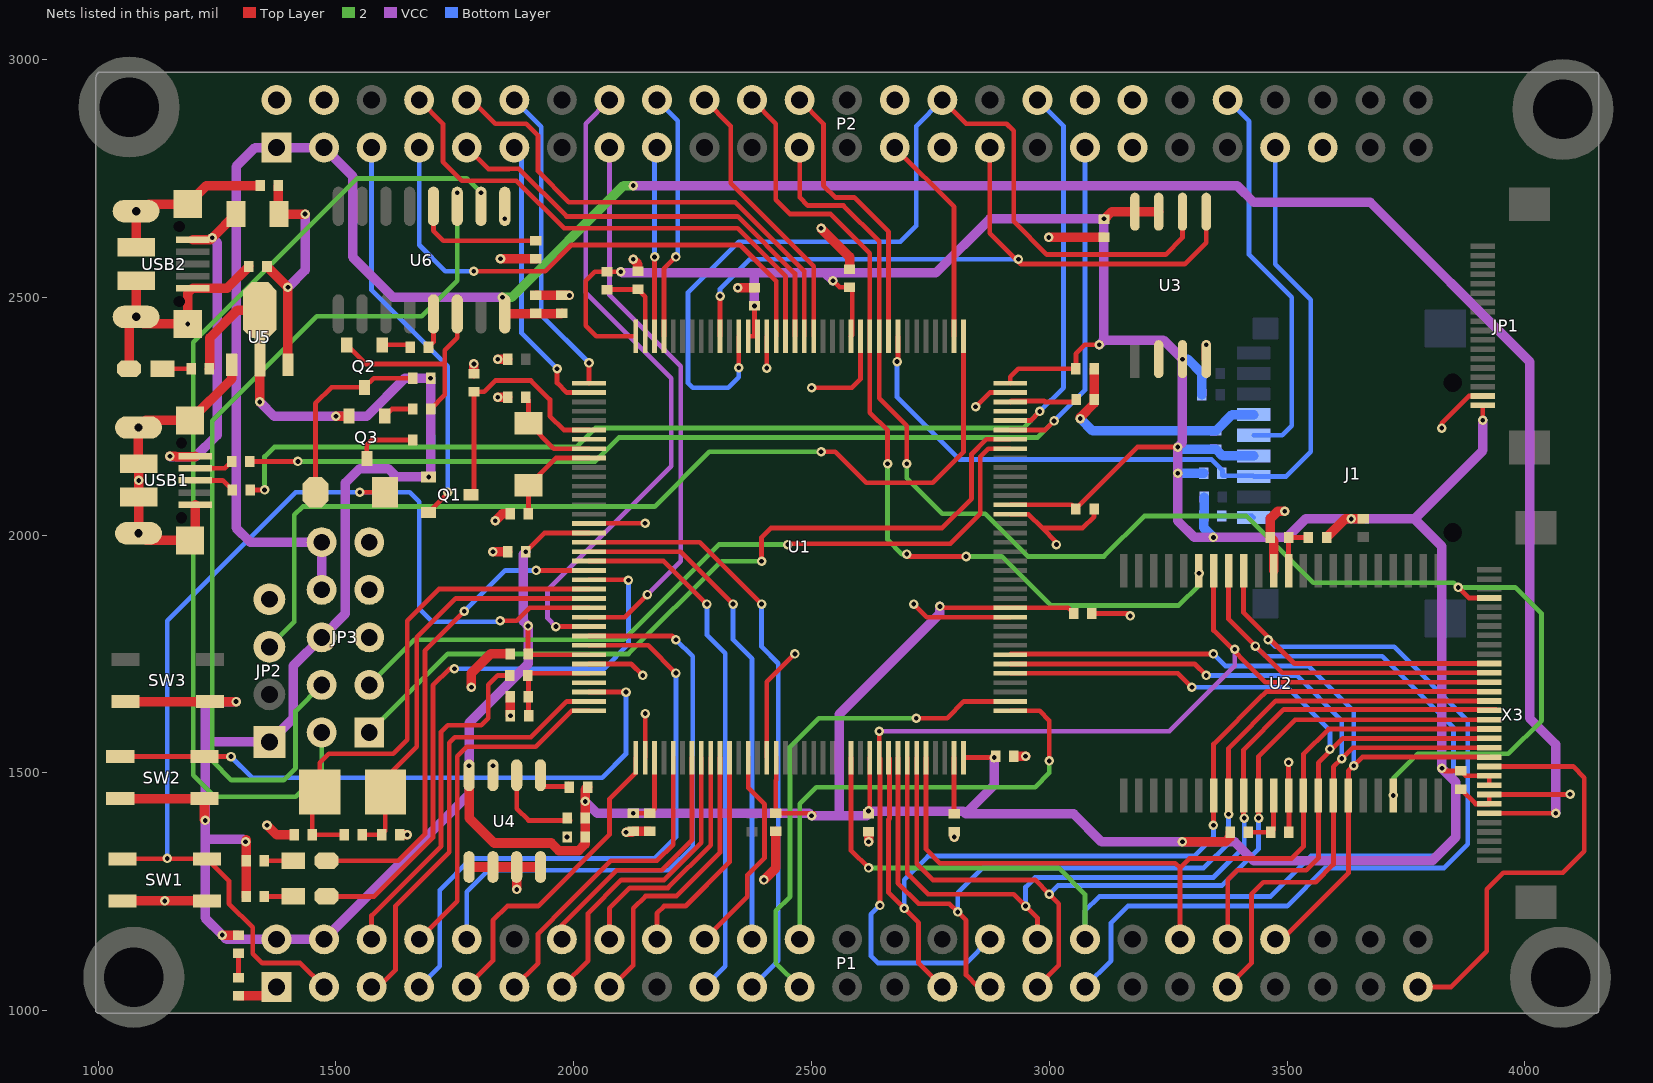
[diagram p0: the nets of this part, all layers, seen from the top]
# Altium PCB MISC105440.PcbDoc (part 2 of 2)
Units mil, origin at the board's own origin, x right, y up, seen from the top; angles counter-clockwise.
Board outline 3160.03 x 1978.53 mil, 4 copper layers (Top Layer, 2, VCC, Bottom Layer), stack 30.634 mil thick; 91 components, 148 nets, 590 pads, 216 vias.

## Via types
v1: diameter 20, hole 10, Top Layer to Bottom Layer, 216 vias

## Nets (pads, with @x,y where several pads share a name; then routed paths per layer and width w, separated by ;. In a path a pad name is that pad's centre, name@x,y a point inside that pad or via, vN(x,y) a via of type N, cw(c..) or ccw(c..) an arc to the next point about the centre after c; other vN are vias at no path point) (continued)
FSMC_D5: P1.35 U2.14 X3.22 | length 2375.7
  Top Layer w10: U2.14@3408.5,1925 3408.5,1836.5 3515,1730 X3.22@3925,1730
  Bottom Layer w10: P1.35@3075,1050 3130,1105 3130,1185 3165,1220 3500,1220 3580,1300 3830,1300 3880,1350 3880,1610 3725,1765 3475,1765 v1(3460,1780)
FSMC_D6: P1.36 U1.60 U2.15 X3.21 | length 3139.6
  Top Layer w10: U1.60@2583.27,1532.09 2583.27,1336.73 v1(2620,1300) ; U2.15@3377.01,1925 3377.01,1822.99 3489.69,1710.31 X3.21@3925,1710.31
  2 w10: v1(2620,1300) 3020,1300 3075,1245 P1.36@3075,1150
  Bottom Layer w10: P1.36@3075,1150 3075,1210 3105,1240 3465,1240 3550,1325 3820,1325 3850,1355 3850,1595 3700,1745 3455,1745 v1(3433.35,1766.65)
FSMC_D7: P1.32 U1.63 U2.16 X3.20 | length 2349.3
  Top Layer w10: v1(2642.32,1587.68) U1.63@2642.32,1532.09 2643.81,1530.6 v1(2643.81,1221.19) v1@2645,1220 ; U2.16@3345.51,1925 3345.51,1799.49 3454.37,1690.63 X3.20@3925,1690.63
  VCC w10: v1(2642.32,1587.68) 3252.68,1587.68 3390,1725 v1(3390,1760)
  Bottom Layer w10: v1(2643.81,1221.19) 2625,1202.38 2625,1115 2640,1100 2825,1100 P1.32@2875,1150
FSMC_D8: P1.29 U1.64 U2.29 X3.19 | length 2098.8
  Top Layer w10: U1.64@2662.01,1532.09 2664,1530.09 2664,1403.85 2662.01,1401.85 2662.01,1247.99 v1(2695,1215) 2725,1185 2725,1100 P1.29@2775,1050 ; v1(3345,1390) 3345.51,1390.51 U2.29@3345.51,1452.56 3345.51,1560.51 3448,1663 3448.54,1663 3456.48,1670.94 X3.19@3925,1670.94
  Bottom Layer w10: v1(2695,1215) 2695,1275 2745,1325 3305,1325 3345,1365 v1(3345,1390)
FSMC_D9: P1.31 U1.65 U2.30 X3.18 | length 2059.3
  Top Layer w10: U1.65@2681.69,1532.09 2681.69,1268.31 2725,1225 2790,1225 v1(2807.5,1207.5) 2825,1190 2825,1075 2850,1050 P1.31@2875,1050 ; v1(3377.01,1412.99) U2.30@3377.01,1452.56 3377.01,1552.01 3476.26,1651.26 X3.18@3925,1651.26
  Bottom Layer w10: v1(2807.5,1207.5) 2807.5,1247.5 2860,1300 3325,1300 3380,1355 3377.01,1357.99 v1(3377.01,1412.99)
FSMC_D10: P1.34 U1.66 U2.31 X3.17 | length 1906.8
  Top Layer w10: U1.66@2701.38,1532.09 2701.38,1288.62 2745,1245 2925,1245 v1(2950,1220) 2975,1195 P1.34@2975,1150 ; v1(3410,1405) 3408.5,1406.5 U2.31@3408.5,1452.56 3408.5,1548.5 3493.35,1633.35 X3.17@3940,1633.35
  Bottom Layer w10: v1(2950,1220) 2950,1260 2970,1280 3345,1280 3410,1345 v1(3410,1405)
FSMC_D11: P1.33 U1.67 U2.32 X3.16 | length 1941.7
  Top Layer w10: U1.67@2721.06,1532.09 2721.06,1308.94 2755,1275 2970,1275 v1(3000,1245) 3020,1225 3020,1095 P1.33@2975,1050 ; v1(3440,1405) U2.32@3440,1452.56 3440,1535 3516.89,1611.89 X3.16@3925,1611.89
  Bottom Layer w10: v1(3000,1245) 3018,1263 3363,1263 3440,1340 v1(3440,1405)
FSMC_D12: P1.40 U1.68 U2.35 X3.15 | length 1778.6
  Top Layer w10: U1.68@2740.75,1532.09 2740.75,1339.25 2770,1310 3265,1310 3275,1300 ; P1.40@3275,1150 3275,1300 ; X3.15@3925,1592.2 3587.2,1592.2 3534.49,1539.49 U2.35@3534.49,1452.56 3534.49,1344.49 3510,1320 3295,1320 3275,1300
FSMC_D13: P1.42 U1.77 U2.36 X3.14 | length 1677.2
  Top Layer w10: U1.77@2917.91,1709.25 2918.28,1709.62 3270.38,1709.62 v1(3300,1680) ; P1.42@3375,1150 3375,1275 3395,1295 3540,1295 3565.98,1320.98 U2.36@3565.98,1452.56 3565.98,1520.98 3617.52,1572.52 X3.14@3925,1572.52
  Bottom Layer w10: v1(3300,1680) 3500,1680 3590,1590 v1(3590,1550)
FSMC_D14: P1.41 U1.78 U2.37 X3.13 | length 1789.7
  Top Layer w10: U1.78@2917.91,1728.94 3306.06,1728.94 v1(3330,1705) ; P1.41@3375,1050 3425,1100 3425,1245 3450,1270 3560,1270 3597.48,1307.48 U2.37@3597.48,1452.56 3597.48,1512.48 v1(3615,1530) 3637.83,1552.83 X3.13@3925,1552.83
  Bottom Layer w10: v1(3330,1705) 3520,1705 3615,1610 v1(3615,1530)
FSMC_D15: P1.44 U1.79 U2.38 X3.12 | length 1622
  Top Layer w10: U1.79@2917.91,1748.62 2919.29,1750 v1(3345,1750) ; P1.44@3475,1150 3490,1150 3628.98,1288.98 U2.38@3628.98,1452.56 3628.98,1503.98 v1(3640,1515) 3658.15,1533.15 X3.12@3925,1533.15
  Bottom Layer w10: v1(3345,1750) 3370,1725 3545,1725 3640,1630 v1(3640,1515)
FSMC_NBL0: P2.18 U1.141 | length 527.1
  Top Layer w10: U1.141@2189.57,2417.91 2189.57,2559.57 v1(2215,2585)
  Bottom Layer w10: P2.18@2175,2915 2218.5,2871.5 2218.5,2588.5 v1(2215,2585)
FSMC_NBL1: P2.17 U1.142 | length 399.2
  Top Layer w10: U1.142@2169.88,2417.91 v1(2169.88,2584.88)
  Bottom Layer w10: v1(2169.88,2584.88) 2169.88,2809.88 P2.17@2175,2815
FSMC_NE3: P2.20 U1.125 | length 592.2
  Top Layer w10: P2.20@2275,2915 2330,2860 2330,2740 2504.53,2565.47 U1.125@2504.53,2417.91
FSMC_NE4: P2.9 U1.127 | length 932.1
  Top Layer w10: P2.9@1775,2815 1820,2770 1864.14,2770 1864.34,2770.2 1884.8,2770.2 1985,2670 2345,2670 2465.16,2549.84 U1.127@2465.16,2417.91
FSMC_NOE: P2.23 U1.118 U2.41 X3.29 | length 3052.6
  Top Layer w10: P2.23@2475,2815 2475,2710 2492,2693 2567,2693 2642.32,2617.68 U1.118@2642.32,2417.91 2642.32,2287.68 2700,2230 v1(2700,2150) ; v1(3860,1890) 3882.2,1867.8 X3.29@3925,1867.8
  2 w10: v1(2700,2150) 2700,2120 2775,2045 2865,2045 2955,1955 3115,1955 3200,2040 3415,2040 3555,1900 3850,1900 v1(3860,1890) 3980,1890 4035,1835 4035,1610 3965,1540 3775,1540 3723.47,1488.47 v1(3723.47,1452.56)
FSMC_NWE: P2.22 U1.119 U2.17 | length 1847.8
  Top Layer w10: P2.22@2375,2915 2425,2865 2425,2705 2455,2675 2540,2675 2622.64,2592.36 U1.119@2622.64,2417.91 2622.64,2257.36 2660,2220 v1(2660,2150) ; v1(2700,1960) 2705,1955 v1(2825,1955)
  2 w10: v1(2660,2150) 2660,1990 2690,1960 v1(2700,1960) ; v1(2825,1955) 2900,1955 3003,1852 3272,1852 3315,1895 v1(3315,1920)
GND: C1.1 C2.1 C3.1 C4.1 C5.2 C6.2 C9.1 C10.1 C11.1 C12.1 C13.1 C14.1 C15.1 C16.1 C17.1 C18.1 C19.1 C20.1 C21.2 C22.2 C23.2 C24.1 C25.2 C26.2 C27.2 C28.1 C29.1 C30.1 C31.1 C34.2 C35.2 C37.1 C38.1 J1.6 JP1.2 JP2.4 JP3.5 JP3.7 JP3.9 LED3.2 P1.1 P2.2 P2.4 R3.2 R7.1 SW1.2 U1.16 U1.31 U1.38 U1.51 U1.83 U1.94 U1.107 U1.120 U1.130 U2.12 U2.34 U3.4 U4.1 U4.2 U4.3 U4.4 U4.7 U5.1 U6.1 USB1.5 USB2.5 X3.7 X3.8 | length 5765.5
  Top Layer w10: U1.31@2032.09,1728.94 2121.06,1728.94 v1(2145,1705) ; U1.16@2032.09,2024.21 2032.87,2025 v1(2150,2025) ; U1.38@2150.2,1532.09 v1(2150.2,1624.8) ; U1.51@2406.1,1532.09 2406.1,1691.1 v1(2465,1750) ; v1(2406.1,2351.1) U1.130@2406.1,2417.91 ; v1(2500,2310) 2585,2310 2602.95,2327.95 U1.120@2602.95,2417.91 ; v1(2715,1855) 2742.64,1827.36 U1.83@2917.91,1827.36 ; v1(2845,2270) 2874.8,2299.8 U1.107@2917.91,2299.8 ; U1.94@2917.91,2043.9 2956.1,2043.9 2985,2015 ; v1(3015,1980) 3015,1985 2985,2015 ; C14.1@3089.59,1835 3165,1835 v1(3170,1830) ; C18.1@3094,2055 3094,2039 3070,2015 2985,2015 ; v1@3500,1525 v1(3502.99,1522.01) U2.34@3502.99,1452.56 3504,1451.55 C25.2@3504,1375 ; v1(3825,2225) 3825,2235 3882.36,2292.36 JP1.2@3911.69,2292.36 ; C37.1@3865,1466 3896.28,1434.72 X3.7@3925,1434.72 X3.8@3925,1454.41 4094.41,1454.41 v1(4095,1455)
  Top Layer w20: SW1.2@1051.42,1230.71 SW1.2@1228.58,1230.71 ; LED3.2@1065,2350 1065,2444 USB2.5@1079.78,2458.78 ; USB2.5@1080.4,2535 1079.78,2534.38 USB2.5@1079.78,2458.78 ; USB2.5@1080.4,2605 1080.4,2670 1106.39,2695.98 USB2.5@1188.43,2695.98 1227.44,2735 C31.1@1341,2735 ; USB1.5@1203.94,2064 1203.94,1999.53 USB1.5@1193.43,1989.02 1100.79,1989.02 1085.4,2004.4 USB1.5@1085.4,2080 USB1.5@1085.4,2150 1084.78,2150.62 USB1.5@1084.78,2226.22 1099.54,2240.98 USB1.5@1193.43,2240.98 1280.94,2328.5 U5.1@1280.94,2358.07 ; C23.2@1295,1031.59 1356.59,1031.59 P1.1@1375,1050 ; C30.1@1317,2565 1271,2519 USB2.5@1198.94,2519 1188.43,2508.49 v1(1188.43,2444.02) 1094.54,2444.02 USB2.5@1079.78,2458.78 ; v1(1355,1390) 1375,1370 C4.1@1412,1370 ; C3.1@1634,1370 v1(1650,1370) ; U4.1@1780,1302.09 U4.2@1830,1302.09 U4.3@1880,1302.09 ; v1(1785,1680) 1785,1710 1825,1750 C11.1@1866,1750 ; C24.1@1790,2339.59 v1(1790,2360) ; v1(1830,1965) C15.1@1861,1965 ; v1(1835,2030) 1850,2045 C1.1@1866,2045 ; v1(1840,2290) C2.1@1861,2290 ; v1(1840,2370) R7.1@1861,2370 ; v1(1846,2581) C38.1@1920,2581 ; C21.2@1866,1660 1867,1659 v1(1867,1620) ; v1(1880,1255) U4.3@1880,1302.09 ; C35.2@1920,2504 C34.2@1975,2504 v1(1991,2504) ; U4.4@1930,1302.09 U4.3@1880,1302.09 ; v1(2110,1375) 2123,1375 C20.1@2125,1377 C9.1@2160,1377 ; v1(2125,2580) 2135,2570 R3.2@2135,2554.59 ; v1(2345,2520) C13.1@2380,2520 ; v1(2400,1275) 2425,1300 C19.1@2425,1377 ; v1(2520,2645) 2580,2585 C10.1@2580,2559 ; v1(2620,1355) C17.1@2620,1376 ; v1(2800,1365) C5.2@2800,1376 ; C16.1@2925,1535 v1(2950,1535) ; v1(2999,2626) C27.2@3115,2626 ; v1(3065,2245) 3065,2247.56 3094.59,2277.15 C6.2@3094.59,2285 3094,2285.6 C12.1@3094,2350 ; U3.4@3330,2370 v1(3330,2400) ; U2.12@3471.5,1925 3471.5,1988.5 C26.2@3465,1995 3465,2035 3480,2050 v1(3495,2050)
  Bottom Layer w20: v1(3065,2245) 3091,2219 C28.1@3350,2219 3384.31,2253.31 J1.6@3430,2253.31
  other v1: 1140,1230.71 1986,1365 1830,1515 1085.4,2115 1855,2665
IIC_SCL: R15.1 U4.6 | length 173.8
  Top Layer w10: U4.6@1880,1476.46 1880,1425 1905,1400 R15.1@1992,1400
IIC_SDA: R16.1 U4.5 | length 61.6
  Top Layer w10: U4.5@1935,1471.46 R16.1@1989.54,1471.46 ; R16.1@1989.54,1476.46 R16.1@1989.54,1471.46 ; R16.1@1991,1470 R16.1@1989.54,1471.46
LCD_BL: P1.49 X3.11 | length 908.9
  Top Layer w10: P1.49@3775,1050 3845,1050 3920,1125 3920,1255 3955,1290 4080,1290 4125,1335 4125,1490 4101.54,1513.46 X3.11@3925,1513.46
LED0: LED1.2 U1.21 | length 1032.3
  Top Layer w10: LED1.2@1480,1315 1630.96,1315 1687,1371.04 1687,1757 v1(1770,1840) ; v1@1920,1925 v1(1920.79,1925.79) U1.21@2032.09,1925.79
  Bottom Layer w10: v1(1770,1840) 1855.79,1925.79 v1(1920.79,1925.79)
LED1: LED2.2 U1.22 | length 1260.2
  Top Layer w10: LED2.2@1480,1240.26 1580.26,1240.26 1704,1364 1704,1684 1739,1719 v1(1749,1719) ; U1.22@2032.09,1906.1 2113.9,1906.1 v1(2115,1905)
  Bottom Layer w10: v1(1749,1719) 2064,1719 2115,1770 v1(2115,1905)
NetC1_2: C1.2 U1.9 X2.2 | length 211.1
  Top Layer w10: C1.2@1904,2045 1905,2046 X2.2@1905,2105.04 1961.97,2162.01 U1.9@2032.09,2162.01
NetC2_2: C2.2 U1.8 X2.1 | length 206.7
  Top Layer w10: C2.2@1899,2290 1905,2284 X2.1@1905,2234.96 1958.27,2181.69 U1.8@2032.09,2181.69
NetC3_2: C3.2 R1.1 U1.24 X1.1 | length 882.6
  Top Layer w10: R1.1@1555,1370 C3.2@1596,1370 1603.9,1377.9 X1.1@1603.9,1460 1603.9,1488.9 1670,1555 1670,1785 1751.73,1866.73 U1.24@2032.09,1866.73
NetC4_2: C4.2 R1.2 U1.23 X1.2 | length 1088.5
  Top Layer w10: R1.2@1517,1370 C4.2@1450,1370 1450,1443.9 X1.2@1466.1,1460 1466.1,1521.1 1485,1540 1620,1540 1650,1570 1650,1820 1716.42,1886.42 U1.23@2032.09,1886.42
NetC5_1: C5.1 U1.71 | length 120.1
  Top Layer w10: C5.1@2795,1413.99 2799.8,1418.79 U1.71@2799.8,1532.09
NetC6_1: C6.1 U1.106 | length 142.3
  Top Layer w10: U1.106@2917.91,2280.12 2919.8,2282 2989.11,2282 2990.99,2280.12 3051.71,2280.12 C6.1@3056.59,2285
NetC23_1: C23.1 R6.1 | length 51.4
  Top Layer w10: C23.1@1295,1069.59 R6.1@1295,1121
NetC38_2: C38.2 U6.4 | length 290.1
  Top Layer w10: U6.4@1705,2706.38 U6.4@1705,2691.38 1705,2640 1726,2619 C38.2@1920,2619
NetD1_2: D1.2 Q2.3 R24.2 | length 413
  Top Layer w10: D1.2@1456.97,2090 1456.97,2276.97 1490.71,2310.71 Q2.3@1560,2310.71 1579.29,2330 R24.2@1661,2330
NetJ1_1: J1.1 R13.2 | length 68.3
  Bottom Layer w10: R13.2@3363,2040 3426.77,2040 J1.1@3430,2036.77
NetLED1_1: LED1.1 R10.1 | length 61
  Top Layer w10: R10.1@1349,1315 LED1.1@1410,1315
NetLED2_1: LED2.1 R11.1 | length 61.1
  Top Layer w10: R11.1@1349,1240 1409.75,1240 LED2.1@1410,1240.26
NetLED3_1: LED3.1 R12.1 | length 61
  Top Layer w10: LED3.1@1135,2350 R12.1@1196,2350
NetQ2_1: Q2.1 R25.2 | length 61.3
  Top Layer w10: Q2.1@1597.4,2400 1651.58,2400 R25.2@1656.59,2395
NetQ2_2: Q2.2 R26.1 U6.14 | length 461
  Top Layer w10: Q2.2@1522.6,2400 1562.6,2360 1728.81,2360 ; R26.1@1699,2265 1728.81,2294.81 1728.81,2360 ; U6.14@1755,2480 U6.14@1755,2465 1755,2415 1728.81,2388.81 1728.81,2360
NetQ3_1: Q3.1 R26.2 | length 64.8
  Top Layer w10: Q3.1@1602.4,2250 1617.4,2265 R26.2@1661,2265
NetQ3_3: Q3.3 R27.1 | length 129.4
  Top Layer w10: Q3.3@1565,2160.71 1565,2190 1575,2200 R27.1@1661,2200
NetR3_1: R3.1 R4.1 U1.143 | length 170.2
  Top Layer w10: R4.1@2070,2516 2070.59,2516.59 R3.1@2135,2516.59 2150.2,2501.39 U1.143@2150.2,2417.91
NetR22_1: R22.1 USB1.2 | length 83.1
  Top Layer w10: USB1.2@1203.94,2140.5 1266.5,2140.5 R22.1@1281,2155
NetR23_1: R23.1 USB1.3 | length 85.9
  Top Layer w10: USB1.3@1203.94,2115 1261.6,2115 R23.1@1281.59,2095
NetR25_1: R25.1 U6.13 | length 89.3
  Top Layer w10: R25.1@1694.59,2395 1705,2405.41 U6.13@1705,2465 U6.13@1705,2480
PA0: SW2.2 U1.34 | length 1311.3
  Top Layer w10: SW2.2@1046.42,1534.29 SW2.2@1223.58,1534.29 v1(1279.29,1534.29) v1@1280,1535 ; U1.34@2032.09,1669.88 v1(2109.88,1669.88)
  Bottom Layer w10: v1(1279.29,1534.29) 1323.58,1490 2060,1490 2109.88,1539.88 v1(2109.88,1669.88)
PA1: P1.5 U1.35 | length 919.5
  Top Layer w10: P1.5@1575,1050 1590,1050 1625,1085 1625,1220 1738,1333 1738,1563 1750,1575 1910,1575 1985.2,1650.2 U1.35@2032.09,1650.2
PA2: P1.8 U1.36 | length 734.8
  Top Layer w10: P1.8@1675,1150 1755,1230 1755,1535 1775,1555 1920,1555 1995.51,1630.51 U1.36@2032.09,1630.51
PA3: P1.9 U1.37 | length 667.4
  Top Layer w10: P1.9@1775,1050 1830,1105 1830,1190 1860,1220 1925,1220 2075,1370 2075,1445 2130.51,1500.51 U1.37@2130.51,1532.09
PA5: P1.11 U1.41 | length 677.4
  Top Layer w10: P1.11@1875,1050 1925,1100 1925,1161.51 1956.98,1193.5 1956.98,1193.98 2078,1315 2175,1315 2209.25,1349.25 U1.41@2209.25,1532.09
PA7: P1.14 U1.43 | length 551.1
  Top Layer w10: P1.14@1975,1150 1975,1180 2090,1295 2185,1295 2248.62,1358.62 U1.43@2248.62,1532.09
PA9: JP3.3 U1.101 | length 1628.9
  Top Layer w10: v1(2450,1980) 2452,1982 2792,1982 2855,2045 2855,2165 2871.69,2181.69 U1.101@2917.91,2181.69
  2 w10: JP3.3@1570,1685 1665,1780 2105,1780 2305,1980 v1(2450,1980) v1@2455,1980
PA10: JP3.1 U1.102 | length 1687.6
  Top Layer w10: v1(2395,1945) 2395,1995 2415,2015 2775,2015 2836.49,2076.49 2836.49,2170.53 2867.34,2201.38 U1.102@2917.91,2201.38
  2 w10: JP3.1@1570,1585 1735,1750 2115,1750 2310,1945 v1(2395,1945)
PA11: P2.35 R22.2 U1.103 | length 2428.1
  Top Layer w10: R22.2@1319,2155 v1(1420,2155) ; U1.103@2917.91,2221.06 2991.06,2221.06 v1(3010,2240)
  2 w10: v1(1420,2155) 2045,2155 2095,2205 2975,2205 v1(3010,2240)
  Bottom Layer w10: v1(3010,2240) 3075,2305 P2.35@3075,2815
PA12: P2.34 R23.2 U1.104 | length 2538.3
  Top Layer w10: R23.2@1319.59,2095 v1(1350,2095) ; U1.104@2917.91,2240.75 2960.75,2240.75 v1(2980,2260)
  2 w10: v1(1350,2095) 1350,2165 1370,2185 2005,2185 2045,2225 2945,2225 v1(2980,2260)
  Bottom Layer w10: P2.34@2975,2915 3030,2860 3030,2310 v1(2980,2260)
PA13: U1.105
PA14: JP2.3 U1.109 | length 2063.2
  Top Layer w10: v1(2520,2175) 2550,2175 2615,2110 2755,2110 2819.49,2174.49 U1.109@2819.49,2417.91
  2 w10: JP2.3@1360,1765 1412.5,1817.5 1412.5,2042.5 1430,2060 2170,2060 2285,2175 v1(2520,2175) v1@2525,2175
PA15: P2.27 U1.110 | length 448.8
  Top Layer w10: P2.27@2675,2815 2799.8,2690.2 U1.110@2799.8,2417.91
PB0: P1.15 U1.46 | length 619.5
  Top Layer w10: P1.15@2075,1050 2080,1050 2125,1095 2125,1215 2151,1241 2216,1241 2307.68,1332.68 U1.46@2307.68,1532.09
PB1: P1.18 U1.47 | length 471.6
  Top Layer w10: P1.18@2175,1150 2175,1205 2190,1220 2235,1220 2327.36,1312.36 U1.47@2327.36,1532.09
PB3: P2.30 U1.133 U3.6 | length 2042.4
  Top Layer w10: v1(2347.05,2352.05) U1.133@2347.05,2417.91 ; P2.30@2775,2915 2825,2865 2910,2865 2925,2850 2925,2660 2995,2590 3245,2590 3280,2625 U3.6@3280,2680
  Bottom Layer w10: v1(2347.05,2352.05) 2347.05,2332.05 2325,2310 2250,2310 2240,2320 2240,2510 2347,2617 2687,2617 2720,2650 2720,2860 P2.30@2775,2915
PB4: U3.2
PB5: P2.31 U1.135 U3.5 | length 1498.5
  Top Layer w10: U1.135@2307.68,2417.91 v1(2307.68,2502.68) ; P2.31@2875,2815 2875,2635 2940,2570 3285,2570 3330,2615 U3.5@3330,2680
  Bottom Layer w10: v1(2307.68,2502.68) 2307.68,2517.68 2370,2580 v1(2935,2580)
PB10: P2.28
PB11: P2.29
PB12: P1.24 U1.73 | length 1037.5
  Top Layer w10: U1.73@2917.91,1630.51 2979.49,1630.51 3000,1610 v1(3000,1525)
  2 w10: P1.24@2475,1150 2475,1435 2510,1470 2970,1470 3000,1500 v1(3000,1525)
PB13: P1.23 U1.74 | length 1040.5
  Top Layer w10: v1(2720,1615) 2785,1615 2820.2,1650.2 U1.74@2917.91,1650.2
  2 w10: P1.23@2475,1050 2425,1100 2425,1210 2455,1240 2455,1555 2515,1615 v1(2720,1615)
PC0: P2.15 U1.26 | length 1173.8
  Top Layer w10: U1.26@2032.09,1827.36 2107.36,1827.36 v1(2155,1875)
  VCC w10: P2.15@2075,2815 2075,2505 2225,2355 2225,1945 v1(2155,1875)
PC1: P2.16 U1.27 | length 1387
  Top Layer w10: v1(1962.68,1807.68) U1.27@2032.09,1807.68
  VCC w10: v1(1962.68,1807.68) 1945,1825.36 1945,1885 2205,2145 2205,2330 2025,2510 2025,2865 P2.16@2075,2915
PC2: P1.10 U1.28 | length 1250.1
  Top Layer w10: U1.28@2032.09,1787.99 2207.01,1787.99 v1(2215,1780)
  Bottom Layer w10: P1.10@1775,1150 1775,1250 1820,1295 2200,1295 2250,1345 2250,1745 v1(2215,1780)
PC3: P1.7 U1.29 | length 1316.3
  Top Layer w10: U1.29@2032.09,1768.31 2156.69,1768.31 v1(2215,1710)
  Bottom Layer w10: P1.7@1675,1050 1718.5,1093.5 1718.5,1253.5 1785,1320 2170,1320 2215,1365 v1(2215,1710)
PC4: P1.13 U1.44 | length 656.3
  Top Layer w10: P1.13@1975,1050 2030,1105 2030,1205 2100,1275 2190,1275 2268.31,1353.31 U1.44@2268.31,1532.09
PC5: P1.16 U1.45 | length 517.2
  Top Layer w10: P1.16@2075,1150 2075,1215 2118,1258 2198,1258 2287.99,1347.99 U1.45@2287.99,1532.09
PC10: P2.45
PC12: J1.5 P2.42 | length 829.2
  Bottom Layer w10: P2.42@3375,2915 3420,2870.01 3420,2590 3510,2500 3510,2230 3490,2210 J1.5@3430,2210
PC13: U1.7
PD2: J1.3 P2.43 R17.2 U1.116 | length 1766.5
  Top Layer w10: v1(2680,2365) 2681.69,2366.69 U1.116@2681.69,2417.91
  Bottom Layer w10: v1(2680,2365) 2680,2290 2811,2159 3341,2159 3364,2136 3364,2125 3428.39,2125 J1.3@3430,2123.39 3498.39,2123.39 3550,2175 3550,2495 3475,2570 P2.43@3475,2815
PD3: P2.24 U1.117 | length 598
  Top Layer w10: P2.24@2475,2915 2525,2865 2525,2735 2550,2710 2590,2710 2662.01,2637.99 U1.117@2662.01,2417.91
PE2: P2.12 U1.1 | length 660.6
  Top Layer w10: U1.1@2032.09,2319.49 v1(2032.09,2362.09)
  Bottom Layer w10: P2.12@1875,2915 1931.5,2858.5 1931.5,2462.67 v1(2032.09,2362.09)
PE3: P2.11 U1.2 | length 607.7
  Top Layer w10: v1(1965,2350) 1965,2320 1985.2,2299.8 U1.2@2032.09,2299.8
  Bottom Layer w10: P2.11@1875,2815 1890,2800 1890,2425 v1(1965,2350)
PF6: P1.21 U1.18 | length 1259
  Top Layer w10: U1.18@2032.09,1984.84 2265.16,1984.84 v1(2395,1855)
  Bottom Layer w10: P1.21@2375,1050 2430,1105 2430,1730 2395,1765 v1(2395,1855)
PF7: P1.22 U1.19 | length 1073.6
  Top Layer w10: U1.19@2032.09,1965.16 2224.84,1965.16 v1(2335,1855) v1@2337.5,1852.5
  Bottom Layer w10: v1(2335,1855) 2335,1780 2375,1740 P1.22@2375,1150
PF8: P1.19 U1.20 | length 1124.3
  Top Layer w10: U1.20@2032.09,1945.47 2189.53,1945.47 v1(2280,1855)
  Bottom Layer w10: P1.19@2275,1050 2318.5,1093.5 2318.5,1751.5 2280,1790 v1(2280,1855)
PF11: P1.20 U1.49 | length 448.6
  Top Layer w10: P1.20@2275,1150 2365,1240 2365,1285 2401.19,1321.19 2401.19,1433.81 2366.73,1468.27 U1.49@2366.73,1532.09
PG6: P2.38
PG7: P2.37
PG8: P2.36
PG11: P2.10 U1.126 | length 1040.1
  Top Layer w10: P2.10@1775,2915 1785,2915 1835,2865 1900,2865 1925,2840 1925,2765 1990,2700 2340,2700 2484.84,2555.16 U1.126@2484.84,2417.91
PG13: P2.8 U1.128 | length 1097.4
  Top Layer w10: P2.8@1675,2915 1725,2865 1725,2785 1765,2745 1879.58,2745 1979.58,2645 2345,2645 2445.47,2544.53 U1.128@2445.47,2417.91
PG14: P2.7 U1.129 | length 1149
  Top Layer w10: v1(1790,2555) 1940,2555 1995,2610 2350,2610 2425.79,2534.21 U1.129@2425.79,2417.91
  Bottom Layer w10: P2.7@1675,2815 1675,2610 1730,2555 v1(1790,2555)
RESET: D1.1 P1.3 SW1.1 U1.25 | length 2403.8
  Top Layer w10: SW1.1@1051.42,1319.29 SW1.1@1228.58,1319.29 1275,1272.87 1275,1225 1325,1175 1325,1120 1345,1100 1425,1100 P1.3@1475,1050 ; v1(1550,2090) D1.1@1603.03,2090 ; v1(1845,1820) 1880,1820 1907.05,1847.05 U1.25@2032.09,1847.05
  Bottom Layer w10: v1(1145,1320) 1145,1820 1415,2090 v1(1550,2090) 1655,2090 1675,2070 1675,1845 1702,1818 1843,1818 v1(1845,1820)
RXD: JP3.4 U6.3 | length 1936.9
  2 w10: JP3.4@1470,1685 1415,1630 1415,1510 1390,1485 1280,1485 1240,1525 1240,2240 1460,2460 1680,2460 1755,2535 v1(1755,2720)
TXD: JP3.2 U6.2 | length 2061.8
  2 w10: JP3.2@1470,1585 1470,1505 1415,1450 1245,1450 1200,1495 1200,2405 1545,2750 1775,2750 v1(1805,2720)
USB_5V: F1.1 USB1.1 USB2.1 | length 705.1
  Top Layer w20: v1(1151,2166) 1162.32,2166 1163.4,2164.93 1203.94,2164.93 USB1.1@1203.94,2166 ; USB2.1@1198.94,2621 1236,2621 v1(1240,2625) F1.1@1290,2675
  VCC w20: v1(1151,2166) 1152.07,2164.93 1204.93,2164.93 1250,2210 1250,2615 v1(1240,2625)
VBAT: P2.5 Q1.2 | length 850.2
  Top Layer w10: Q1.2@1695,2047.6 1735,2087.6 v1(1735,2090)
  Bottom Layer w10: P2.5@1575,2815 1575,2515 1735,2355 v1(1735,2090)
VBAT_IN: C24.2 Q1.3 U1.6 | length 534.3
  Top Layer w10: Q1.3@1784.29,2085 1790,2090.71 C24.2@1790,2301.59 1811.59,2301.59 1835,2325 1910,2325 1950,2285 1950,2250 1978.94,2221.06 U1.6@2032.09,2221.06
VCC3.3: C9.2 C10.2 C11.2 C12.2 C13.2 C14.2 C15.2 C16.2 C17.2 C18.2 C19.2 C20.2 C27.1 C28.2 C29.2 C37.2 J1.4 JP1.1 JP2.1 JP3.6 P1.2 P1.4 Q1.1 Q3.2 R4.2 R6.2 R9.2 R10.2 R11.2 R12.2 R13.1 R14.1 R15.2 R16.2 R17.1 R18.1 R19.1 R20.1 R21.1 R24.1 SW2.1 SW3.1 U1.17 U1.30 U1.39 U1.52 U1.62 U1.72 U1.84 U1.95 U1.108 U1.121 U1.131 U1.132 U1.144 U3.3 U3.7 U3.8 U4.8 U5.2 X3.9 X3.10 | length 14113.3
  Top Layer w10: v1(1899,1965) 1938.53,2004.53 U1.17@2032.09,2004.53 ; v1(1904,1809) C11.2@1904,1750 1905.38,1748.62 U1.30@2032.09,1748.62 ; v1(2099,2554) R4.2@2070,2554 2044,2554 2025,2535 2025,2440 2047.09,2417.91 U1.144@2130.51,2417.91 ; v1(2125,1415) C9.2@2160,1415 2169.88,1424.88 U1.39@2169.88,1532.09 ; U1.132@2366.73,2417.91 U1.131@2386.42,2417.91 2380,2424.33 v1(2380,2482) ; U1.52@2425.79,1532.09 2425.79,1485 2425,1484.21 C19.2@2425,1415 v1@2505,1415 ; v1(2545,2535) 2559,2521 C10.2@2580,2521 2585.58,2515.42 2585.58,2420.23 U1.121@2583.27,2417.91 ; v1(2620,1420) 2622.64,1422.64 U1.62@2622.64,1532.09 ; v1(2770,1850) 2772.95,1847.05 U1.84@2917.91,1847.05 3039.54,1847.05 C14.2@3051.59,1835 ; U1.72@2819.49,1532.09 v1(2884.09,1532.09) ; U1.95@2917.91,2063.58 3047.42,2063.58 C18.2@3056,2055 3056,2055.78 3185.22,2185 v1(3270,2185) ; U1.108@2917.91,2319.49 2917.91,2332.91 2935,2350 C12.2@3056,2350 3056,2381 3075,2400 v1(3105,2400) ; v1(3825.5,1509.5) 3831,1504 C37.2@3865,1504 3875.22,1493.78 X3.10@3925,1493.78 X3.9@3925,1474.09 ; v1(3911.69,2241.69) JP1.1@3911.69,2272.68
  Top Layer w20: SW2.1@1046.42,1445.71 SW2.1@1223.58,1445.71 v1@1223.58,1401.42 ; SW3.1@1057.83,1650 SW3.1@1235,1650 v1(1290,1650) ; R12.2@1234,2350 1234.95,2350.95 1234.95,2414.95 1293,2473 U5.2@1340,2473 ; v1(1261,1159) R6.2@1295,1159 ; R11.2@1311,1240 R10.2@1311,1315 v1@1311,1359 ; v1(1340,2280) U5.2@1340,2375 ; v1(1500,2250) Q3.2@1527.6,2250 ; U4.8@1780,1495 1780,1405 1832.45,1352.55 1952.6,1352.55 1968.96,1336.19 2010.08,1336.19 2024,1350.11 C29.2@2024,1365 R15.2@2024,1405 v1(2024,1440) 2024,1465 R16.2@2029,1470 ; C27.1@3115,2664 3131,2680 U3.8@3180,2680 U3.7@3230,2680 ; v1(3280,1355) 3370,1355 3380,1365 R21.1@3380,1375 ; R19.1@3583,1995 3622,2034 v1(3635,2034) R9.2@3660,2034
  VCC w20: v1(1290,1650) 1240,1650 1225,1635 1225,1570 ; v1(1310,1355) 1305,1360 1225,1360 ; v1(1340,2280) 1370,2250 v1(1500,2250) 1565,2250 1645,2330 v1(1699,2330) 1699,2126.4 v1(1695,2122.4) 1627.6,2122.4 1610,2140 1550,2140 1520,2110 1520,1835 JP3.6@1470,1785 1410,1725 1410,1686.83 1410.46,1686.37 1410.46,1615.46 JP2.1@1360,1565 1230,1565 1225,1570 ; v1(1899,1965) 1893.79,1959.79 1893.79,1819.21 v1(1904,1809) 1904,1729 1780,1605 v1(1780,1515) 1780,1455 P1.4@1475,1150 P1.2@1375,1150 1270,1150 v1(1261,1159) 1225,1195 1225,1360 ; v1(2024,1440) 2049,1415 v1(2125,1415) 2495,1415 v1(2500,1410) 2558,1410 ; v1(2099,2554) 2101.69,2551.31 2380,2551.31 ; v1(2380,2482) 2380,2551.31 ; v1(2545,2535) 2528.69,2551.31 ; v1(2620,1420) v1@2624,1420 ; v1(2770,1850) 2770,1835 2558,1623 2558,1410 ; v1(2884.09,1532.09) 2884.09,1474.09 2824,1414 ; v1(3105,2400) 3115,2410 ; v1(3911.69,2241.69) 3911.69,2177.91 3767.78,2034 ; 1225,1360 v1(1225,1400) 1225,1570 ; 2380,2551.31 2528.69,2551.31 ; 2528.69,2551.31 2761.31,2551.31 2875,2665 v1(3115,2665) 3115,2410 ; 2558,1410 2616,1410 2625,1419 2819,1419 2824,1414 ; 2824,1414 3051,1414 3110,1355 v1(3280,1355) 3390,1355 3430,1315 3805,1315 3855,1365 3855,1480 v1(3825.5,1509.5) 3825.5,1976.28 3767.78,2034 ; 3115,2410 3240,2410 v1(3280,2370) 3280,2195 v1(3270,2185) v1(3270,2130) 3270,2030 3305,1995 v1(3345,1995) 3500,1995 3539,2034 v1(3635,2034) 3767.78,2034
  Bottom Layer w20: v1(3270,2130) R17.1@3325,2130 ; v1(3270,2185) 3274,2181 C28.2@3350,2181 3350.11,2181 3364.42,2166.69 J1.4@3430,2166.69 ; v1(3280,2370) 3291,2370 R20.1@3321,2340 R18.1@3321,2295 ; R14.1@3326,2080 3326,2041 R13.1@3325,2040 3325,2015 v1(3345,1995)
VCC5: C34.1 C35.1 JP3.8 JP3.10 P2.1 P2.3 U6.16 X3.6 | length 5532.8
  Top Layer w10: X3.6@3925,1415.04 v1(4064.96,1415.04)
  Top Layer w20: U6.16@1855,2495 U6.16@1855,2465 1974,2465 C34.1@1975,2466
  VCC w20: JP3.8@1470,1885 JP3.10@1470,1985 1320,1985 1290,2015 1290,2775 1330,2815 P2.1@1375,2815 P2.3@1475,2815 1535,2755 1535,2585 1620,2500 v1(1850,2500) ; v1(2125,2735) 3395,2735 3430,2700 3675,2700 4010,2365 4010,1615 4064.96,1560.04 v1(4064.96,1415.04)
  2 w20: v1(1850,2500) 1870,2500 2105,2735 v1(2125,2735)
VCC5V: C30.2 C31.2 F1.2 U5.3 | length 509.5
  Top Layer w10: F1.2@1379,2676 F1.2@1380,2675
  Top Layer w20: C30.2@1355,2565 v1(1399.06,2520.94) U5.3@1399.06,2358.07 ; F1.2@1379,2676 C31.2@1379,2735 ; F1.2@1380,2675 v1(1435,2675)
  VCC w20: v1(1399.06,2520.94) 1435,2556.89 v1(1435,2675)
VDDA: U1.33
VREF: P1.6 R5.1 | length 731.2
  Top Layer w10: P1.6@1575,1150 1575,1200 1721,1346 1721,1586 1735,1600 1805,1600 1820,1615 1820,1685 1840,1705 R5.1@1865.41,1705
VREF+: C21.1 C22.1 R5.2 U1.32 | length 216.1
  Top Layer w10: C22.1@1905,1620 1905,1703.41 R5.2@1903.41,1705 1907.66,1709.25 U1.32@2032.09,1709.25
VS1: C26.1 R19.2 U2.11 | length 112
  Top Layer w10: U2.11@3502.99,1925 C26.1@3503,1995 R19.2@3545,1995
VS2: C25.1 R21.2 U2.33 | length 127.8
  Top Layer w10: R21.2@3418,1375 C25.1@3466,1375 3471.5,1380.5 U2.33@3471.5,1452.56
pads on no net: HOLE1.0 HOLE2.0 HOLE3.0 HOLE4.0 J1.0 J1.9 J1.10 JP1.0 JP1.3 JP1.5 JP2.2 P1.37 P2.6 R8.1 R9.1 U1.15 U1.42 U1.53 U1.59 U1.61 U1.69 U1.70 U1.75 U1.76 U1.87 U1.90 U1.91 U1.92 U1.93 U1.111 U1.113 U1.134 U1.139 U1.140 U2.6 U2.39 U2.40 U6.7 U6.8 U6.9 U6.10 U6.11 U6.12 U6.15 USB1.4 USB2.4 X3.0 X3.1 X3.2 X3.3 X3.4 X3.5 X3.28 X3.30 X3.32

## Polygon pours and split planes (outlines as drawn)
GND on Top Layer "D" (solid, remove dead copper, pour order 12): 825,3095 4230,3095 4255,3070 4225,3040 4225,885 960,885 925,850
GND on Bottom Layer "D" (solid, remove dead copper, pour order 14): 790,3120 840,3170 4495,3170 4495,915 4290,710 4225,775 940,775

## Keep-outs
Keep-Out Layer:
  lines w10: 1000,1000 1000,2960.15 cw(c1011.81,2960.15) 1003.46,2968.5 4149.61,2968.5 cw(c4148.66,2967.55) 4150,2967.55 4150,1000 1000,1000